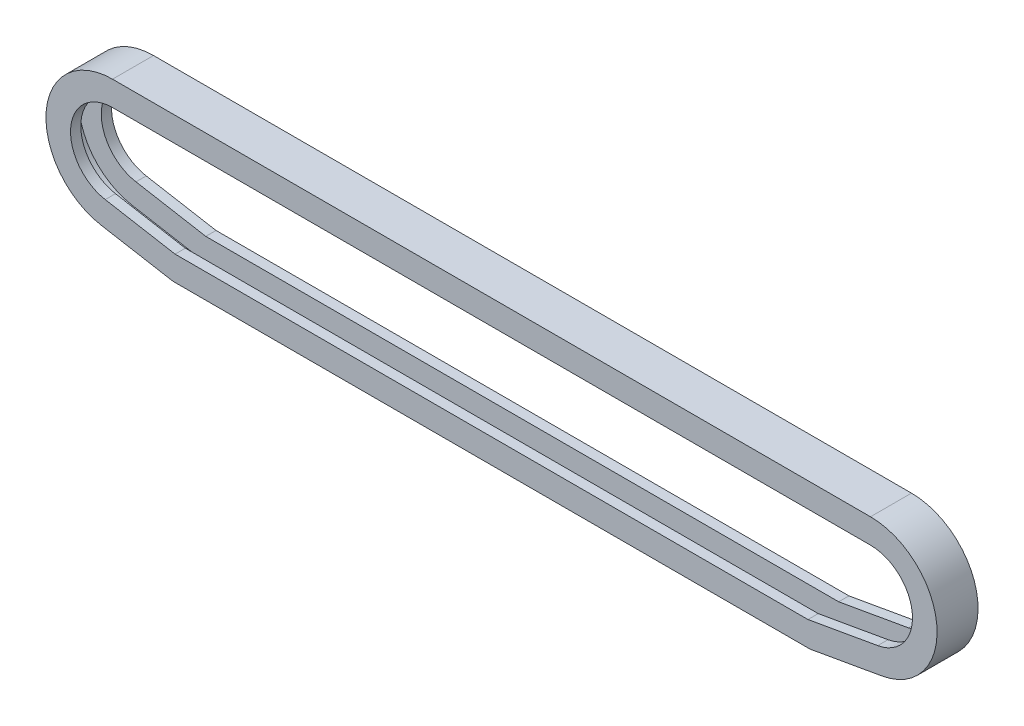
SolidWorks part; units mm, degrees
ref_plane "Front Plane" through (0, 0, 0) normal (0, 0, 1) x (1, 0, 0)
ref_plane "Top Plane" through (0, 0, 0) normal (0, 1, 0) x (1, 0, 0)
ref_plane "Right Plane" through (0, 0, 0) normal (1, 0, 0) x (0, 0, -1)
sketch "Sketch2" plane through (0, 0, 0) normal (0, 0, 1) x (1, 0, 0)
  line L0 (185, 0) -> (-185, 0) construction
  line L1 (0, 0) -> (0, -32.1986) construction
  line L2 (-155, -32.1986) -> (-189.6017, -26.0974) construction
  line L3 (155, -32.1986) -> (189.6017, -26.0974) construction
  line L4 (-185, 26.5) -> (185, 26.5) construction
  line L5 (-155, -32.1986) -> (155, -32.1986) construction
  line L6 (-185, 0) -> (-189.6017, -26.0974) construction
  line L7 (-185, 32.5) -> (185, 32.5)
  line L8 (155.5249, -38.1986) -> (190.6436, -32.0063)
  line L9 (-155.5249, -38.1986) -> (155.5249, -38.1986)
  line L10 (-155.5249, -38.1986) -> (-190.6436, -32.0063)
  line L11 (-185, 20.5) -> (185, 20.5)
  line L12 (154.4751, -26.1986) -> (188.5598, -20.1886)
  line L13 (-154.4751, -26.1986) -> (154.4751, -26.1986)
  line L14 (-154.4751, -26.1986) -> (-188.5598, -20.1886)
  arc A0 (-185, 26.5) -> (-189.6017, -26.0974) centre (-185, 0) ccw construction
  arc A1 (185, 26.5) -> (189.6017, -26.0974) centre (185, 0) cw construction
  arc A2 (185, 32.5) -> (190.6436, -32.0063) centre (185, 0) cw
  arc A3 (-185, 32.5) -> (-190.6436, -32.0063) centre (-185, 0) ccw
  arc A4 (185, 20.5) -> (188.5598, -20.1886) centre (185, 0) cw
  arc A5 (-185, 20.5) -> (-188.5598, -20.1886) centre (-185, 0) ccw
  point P6 (0, 0)
  dimension "D1" = 53
  dimension "D7" = 32.5
  dimension "D8" = 20.5
  dimension "D2" = 370
  dimension "D3" = 30
  dimension "D4" = 100
  dimension "D5" = 6
  dimension "D6" = 6
extrude "Boss-Extrude1" add sketch "Sketch2" along normal mid plane 20
sketch "Sketch8" plane through (0, 0, 0) normal (0, 0, 1) x (1, 0, 0)
  line L18 (155.4374, -37.1986) -> (190.4699, -31.0214)
  line L19 (-155.4374, -37.1986) -> (155.4374, -37.1986)
  line L20 (-190.4699, -31.0214) -> (-155.4374, -37.1986)
  line L21 (185, 31.5) -> (-185, 31.5)
  line L22 (155.4374, -37.1986) -> (190.4699, -31.0214)
  line L23 (-155.4374, -37.1986) -> (155.4374, -37.1986)
  line L24 (-190.4699, -31.0214) -> (-155.4374, -37.1986)
  line L25 (185, 31.5) -> (-185, 31.5)
  arc A12 (190.4699, -31.0214) -> (185, 31.5) centre (185, 0) ccw
  arc A13 (-185, 31.5) -> (-190.4699, -31.0214) centre (-185, 0) ccw
  arc A14 (190.4699, -31.0214) -> (185, 31.5) centre (185, 0) ccw
  arc A15 (-185, 31.5) -> (-190.4699, -31.0214) centre (-185, 0) ccw
  dimension "D1" = 1
extrude "Cut-Extrude1" cut sketch "Sketch8" against normal mid plane 10
